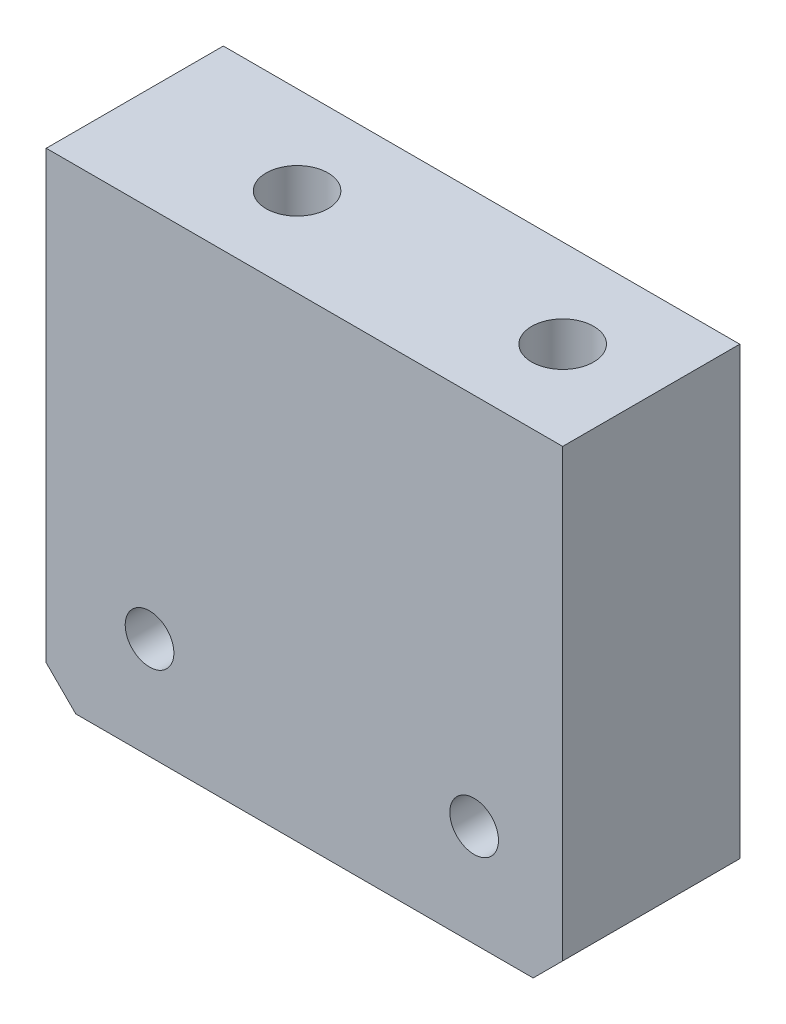
from build123d import *

# Parameters (mm, degrees)
SKETCH1_W             = 35
SKETCH1_H             = 12
BOSS_EXTRUDE1_DEPTH   = 32.2
M5_TAPPED_HOLE1_D     = 4.2
M5_TAPPED_HOLE1_DEPTH = 12.4
M5_TAPPED_HOLE1_TIP   = 1.2618073
CHAMFER2_SIZE         = 2
M4_TAPPED_HOLE1_D     = 3.3


with BuildPart() as part:
    # Sketch1 → Boss-Extrude1 (new body)
    with BuildSketch(Plane(origin=(0, 0, 0), x_dir=(1, 0, 0), z_dir=(0, 1, 0))):
        Rectangle(SKETCH1_W, SKETCH1_H)
    extrude(amount=BOSS_EXTRUDE1_DEPTH)

    # M5 Tapped Hole1
    with Locations(Plane(origin=(11.5, 32.2, 0), x_dir=(0, 0, 1), z_dir=(0, 1, 0))):
        with Locations((0, 0), (0, -18)):
            Hole(M5_TAPPED_HOLE1_D / 2, depth=M5_TAPPED_HOLE1_DEPTH)
            with Locations((0, 0, -(M5_TAPPED_HOLE1_DEPTH + M5_TAPPED_HOLE1_TIP / 2))):  # 118° drill point
                Cone(0, M5_TAPPED_HOLE1_D / 2, M5_TAPPED_HOLE1_TIP, mode=Mode.SUBTRACT)

    # Chamfer2
    chamfer2_edges = [part.edges().sort_by_distance(p)[0] for p in [
        (-17.5, 0, 0),
        (17.5, 0, 0),
    ]]
    chamfer(chamfer2_edges, length=CHAMFER2_SIZE)

    # M4 Tapped Hole1 (through all)
    with Locations(Plane(origin=(11.5, 6.9, -6), x_dir=(-1, 0, 0), z_dir=(0, 0, -1))):
        with Locations((0, 0), (22, 0)):
            Hole(M4_TAPPED_HOLE1_D / 2)


solid = part.part
